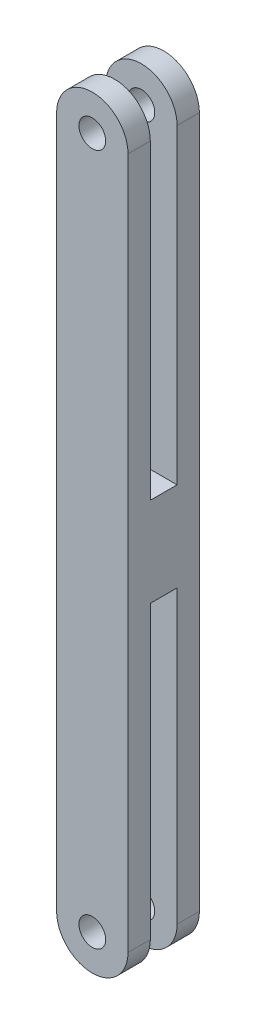
SolidWorks part; units mm, degrees
ref_plane "Front Plane" through (0, 0, 0) normal (0, 0, 1) x (1, 0, 0)
ref_plane "Top Plane" through (0, 0, 0) normal (0, 1, 0) x (1, 0, 0)
ref_plane "Right Plane" through (0, 0, 0) normal (1, 0, 0) x (0, 0, -1)
other "Configuration Table"
sketch "Sketch1" plane through (0, 0, 0) normal (0, 0, 1) x (1, 0, 0)
  line L2 (-8, 79.7267) -> (-8, -75.2733)
  line L4 (8, 79.7267) -> (8, -75.2733)
  line L5 (-7.7059, 81.8757) -> (7.3761, -78.3707) construction
  line L6 (-7.3761, -78.3707) -> (7.7059, 81.8757) construction
  circle A0 centre (0, 79.7267) radius 3
  arc A1 (8, 79.7267) -> (-8, 79.7267) centre (0, 79.7267) ccw
  circle A2 centre (0, -75.2733) radius 3
  arc A3 (-8, -75.2733) -> (8, -75.2733) centre (0, -75.2733) ccw
  point P0 (0, 0)
  dimension "D3" = 155
  dimension "D1" = 6
  dimension "D2" = 6
extrude "Boss-Extrude1" add sketch "Sketch1" along normal blind 16
sketch "Sketch2" plane through (8, 0, 0) normal (1, 0, 0) x (0, 0, -1)
  line L0 (-16, 79.7267) -> (0, 79.7267) construction
  line L1 (-11, 149.4534) -> (-5, 149.4534)
  line L2 (-11, 149.4534) -> (-11, 10)
  line L3 (-11, 10) -> (-5, 10)
  line L4 (-5, 149.4534) -> (-5, 10)
  line L5 (-11, 149.4534) -> (-5, 10) construction
  line L6 (-11, 10) -> (-5, 149.4534) construction
  line L7 (-16, -83.2733) -> (0, -83.2733) construction
  line L8 (-11, -156.5466) -> (-5, -156.5466)
  line L9 (-11, -156.5466) -> (-11, -10)
  line L10 (-11, -10) -> (-5, -10)
  line L11 (-5, -156.5466) -> (-5, -10)
  line L12 (-11, -156.5466) -> (-5, -10) construction
  line L13 (-11, -10) -> (-5, -156.5466) construction
  point P0 (-8, 79.7267)
  point P7 (-8, -83.2733)
  dimension "D1" = 20
  dimension "D2" = 10
  dimension "D3" = 6
  dimension "D4" = 6
extrude "Cut-Extrude1" cut sketch "Sketch2" against normal through all
